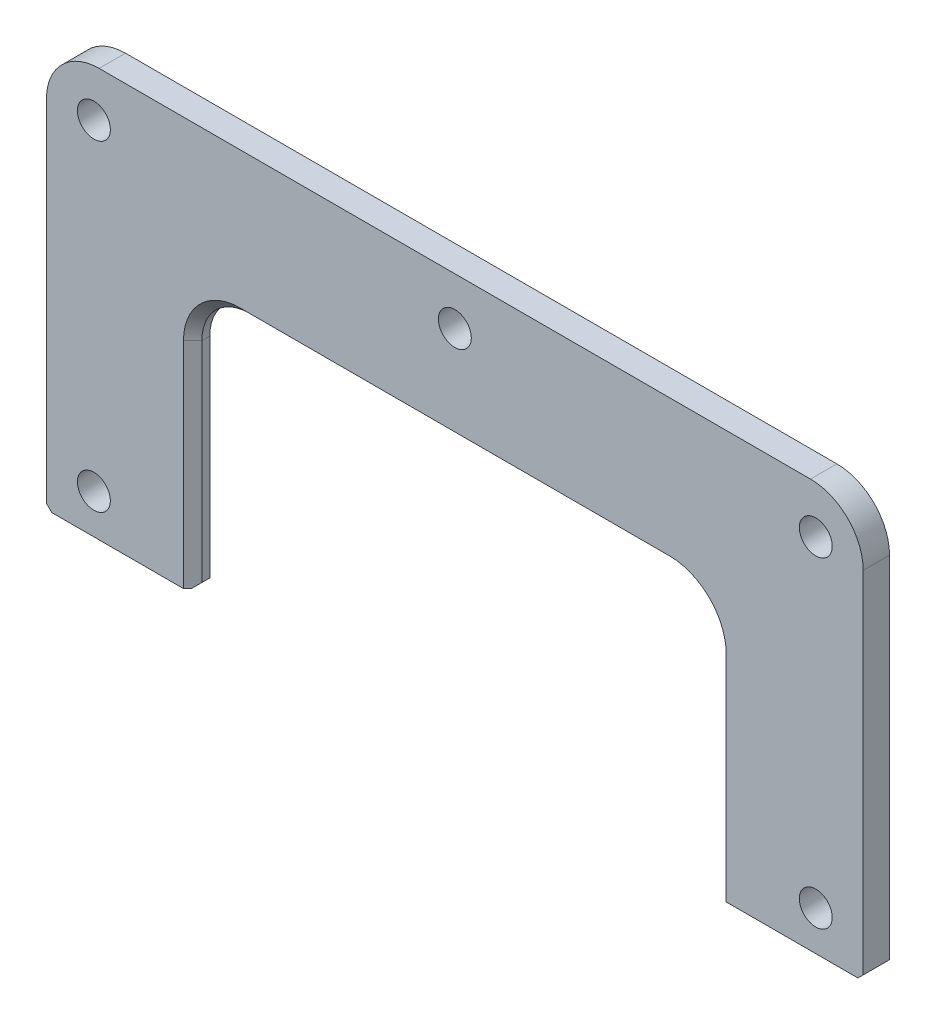
from build123d import *

# Parameters (mm, degrees)
EXTRUDE_1_DEPTH     = 10
SKETCH_2_R          = 6.25
CUT_EXTRUDE_1_DEPTH = 220.431082575
CHAMFER_1_SIZE      = 2
CHAMFER_2_SIZE      = 3.5


with BuildPart() as part:
    # 草图1 → 凸台-拉伸1 (new body)
    with BuildSketch(Plane.XY):
        with BuildLine():
            Line((-155, 0), (-99.5, 0))
            Line((-99.5, 0), (-99.5, 2.5))
            Line((-99.5, 2.5), (-99.5, 81.5))
            ThreePointArc((-99.5, 81.5), (-94.227922061, 94.227922061), (-81.5, 99.5))
            Line((-81.5, 99.5), (81.5, 99.5))
            ThreePointArc((81.5, 99.5), (94.227922061, 94.227922061), (99.5, 81.5))
            Line((99.5, 81.5), (99.5, 2.5))
            Line((99.5, 2.5), (99.5, 0))
            Line((99.5, 0), (155, 0))
            Line((155, 0), (155, 2.5))
            Line((155, 2.5), (155, 135))
            ThreePointArc((155, 135), (149.142135624, 149.142135624), (135, 155))
            Line((135, 155), (-135, 155))
            ThreePointArc((-135, 155), (-149.142135624, 149.142135624), (-155, 135))
            Line((-155, 135), (-155, 2.5))
            Line((-155, 2.5), (-155, 0))
        make_face()
    extrude(amount=EXTRUDE_1_DEPTH)

    # 草图2 → 切除-拉伸1 (cut, through all)
    with BuildSketch(Plane.XY.offset(10)):
        with Locations((0, 137)):
            Circle(SKETCH_2_R)
        with Locations((0, -137)):
            Circle(SKETCH_2_R)
        with Locations((-137, 137)):
            Circle(SKETCH_2_R)
        with Locations((137, 137)):
            Circle(SKETCH_2_R)
        with Locations((-137, -137)):
            Circle(SKETCH_2_R)
        with Locations((137, -137)):
            Circle(SKETCH_2_R)
        with Locations((-137, 15)):
            Circle(SKETCH_2_R)
        with Locations((-137, -15)):
            Circle(SKETCH_2_R)
        with Locations((137, -15)):
            Circle(SKETCH_2_R)
        with Locations(Location((137, 15, 0), (0, 0, 180))):
            Circle(SKETCH_2_R)
    extrude(amount=-CUT_EXTRUDE_1_DEPTH, mode=Mode.SUBTRACT)

    # 倒角1
    chamfer_1_edges = [part.edges().sort_by_distance(p)[0] for p in [
        (-99.5, 0, 5),
        (-155, 0, 5),
        (155, 0, 5),
        (99.5, 0, 5),
    ]]
    chamfer(chamfer_1_edges, length=CHAMFER_1_SIZE)

    # 倒角2
    chamfer_2_edges = [part.edges().sort_by_distance(p)[0] for p in [
        (99.5, 41.75, 0),
        (94.227922061, 94.227922061, 0),
        (0, 99.5, 0),
        (-94.227922061, 94.227922061, 0),
        (-99.5, 41.75, 0),
        (99.5, 41.75, 10),
        (94.227922061, 94.227922061, 10),
        (-99.5, 41.75, 10),
        (-94.227922061, 94.227922061, 10),
        (0, 99.5, 10),
    ]]
    chamfer(chamfer_2_edges, length=CHAMFER_2_SIZE)


solid = part.part
